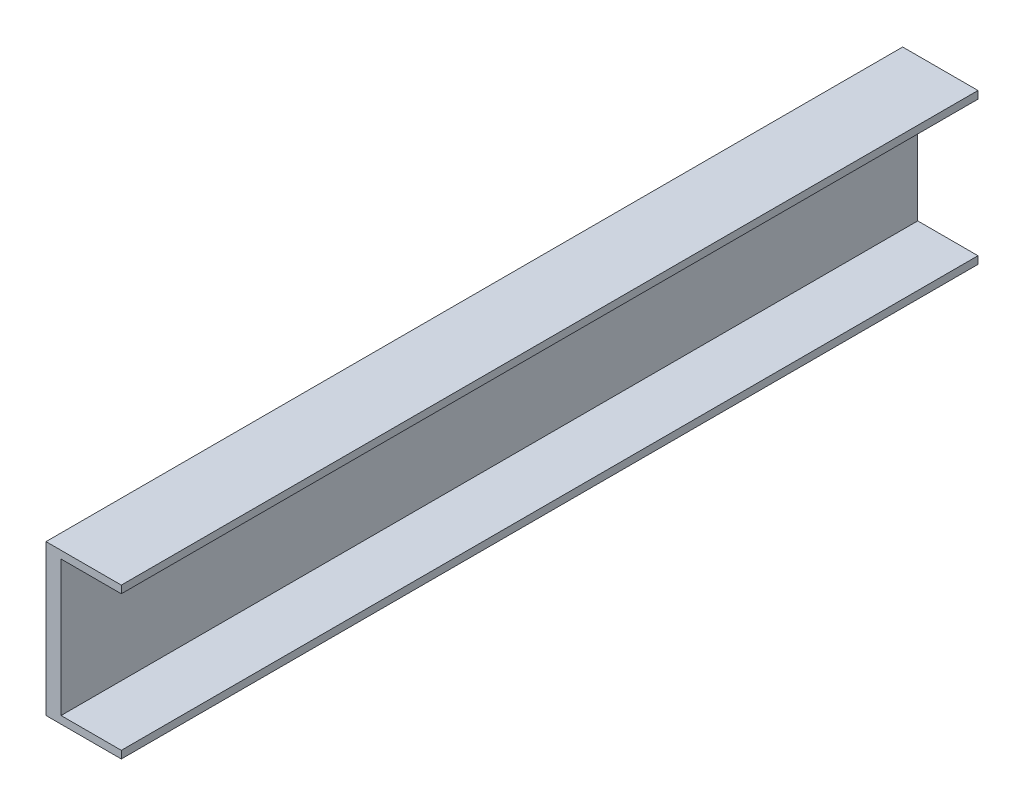
from build123d import *

# Parameters (mm, degrees)
EXTRUDE1_DEPTH = 455


with BuildPart() as part:
    # Sketch1 → Extrude1 (new body)
    with BuildSketch(Plane.XY):
        Polygon((0, 0), (-40, 0), (-40, 80), (0, 80), (0, 76), (-32, 76), (-32, 4), (0, 4), align=None)
    extrude(amount=EXTRUDE1_DEPTH)


solid = part.part
